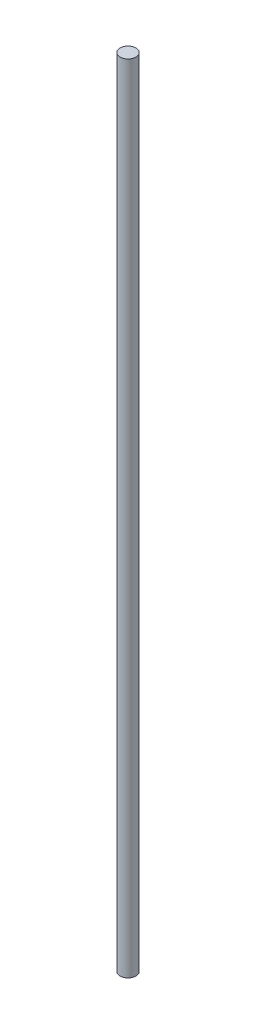
from build123d import *

# Parameters (mm, degrees)
SKETCH1_R           = 10
BOSS_EXTRUDE1_DEPTH = 1000


with BuildPart() as part:
    # Sketch1 → Boss-Extrude1 (new body)
    with BuildSketch(Plane(origin=(0, 0, 0), x_dir=(1, 0, 0), z_dir=(0, 1, 0))):
        with Locations(Location((0, 0, 0), (0, 0, 270))):
            Circle(SKETCH1_R)
    extrude(amount=BOSS_EXTRUDE1_DEPTH)


solid = part.part
